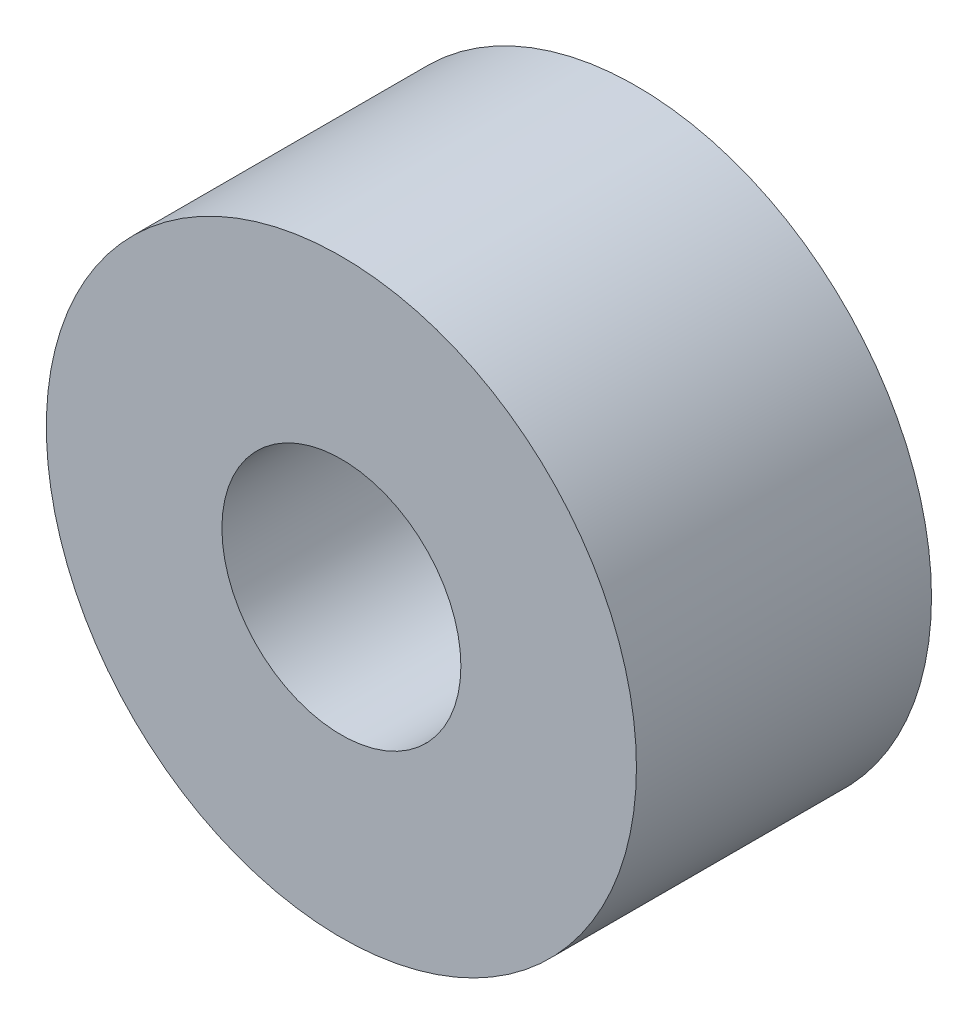
from build123d import *

# Parameters (mm, degrees)
SKETCH_1_R      = 20
SKETCH_1_R_2    = 8.1
EXTRUDE_1_DEPTH = 10


with BuildPart() as part:
    # 草图1 → 凸台-拉伸1 (new, symmetric)
    with BuildSketch(Plane.XY):
        Circle(SKETCH_1_R)
        Circle(SKETCH_1_R_2, mode=Mode.SUBTRACT)
    extrude(amount=EXTRUDE_1_DEPTH, both=True)


solid = part.part
